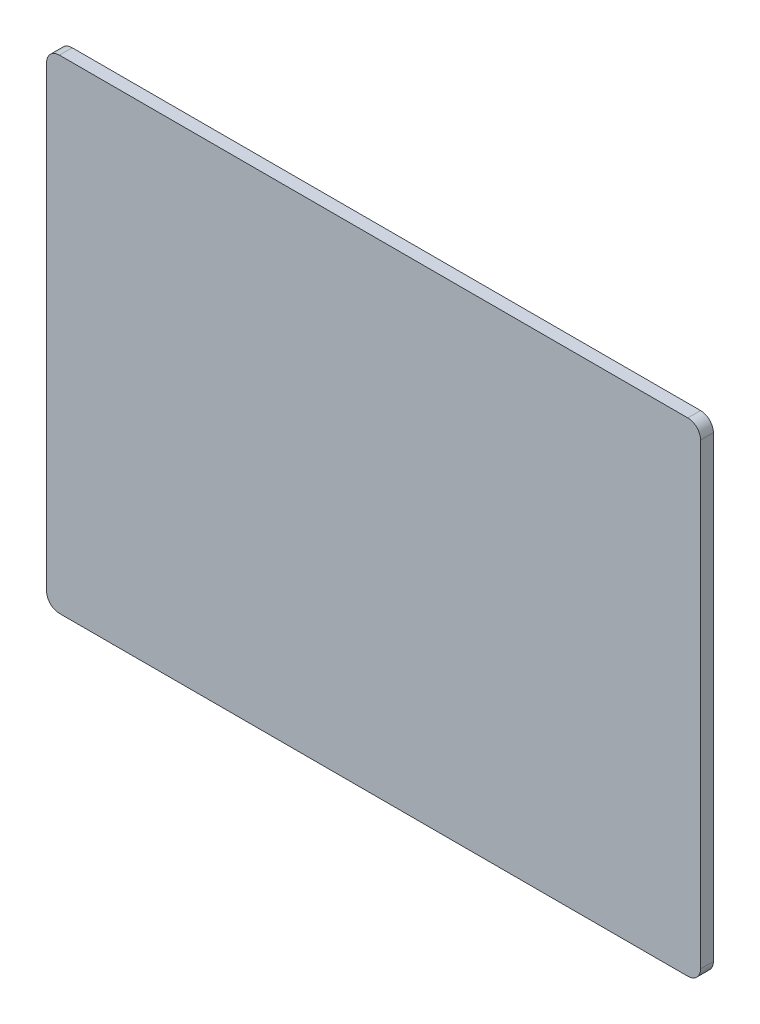
from build123d import *

# Parameters (mm, degrees)
SKETCH_1_W      = 153.5
SKETCH_1_H      = 113.5
EXTRUDE_1_DEPTH = 3
FILLET_1_R      = 3


with BuildPart() as part:
    # 草图1 → 凸台-拉伸1 (new body)
    with BuildSketch(Plane.XY):
        with Locations((109.383738602, -6.302431611)):
            Rectangle(SKETCH_1_W, SKETCH_1_H)
    extrude(amount=EXTRUDE_1_DEPTH)

    # 圆角1
    fillet_1_edges = [part.edges().sort_by_distance(p)[0] for p in [
        (32.633738602, 50.447568389, 1.5),
        (186.133738602, 50.447568389, 1.5),
        (186.133738602, -63.052431611, 1.5),
        (32.633738602, -63.052431611, 1.5),
    ]]
    fillet(fillet_1_edges, radius=FILLET_1_R)


solid = part.part
